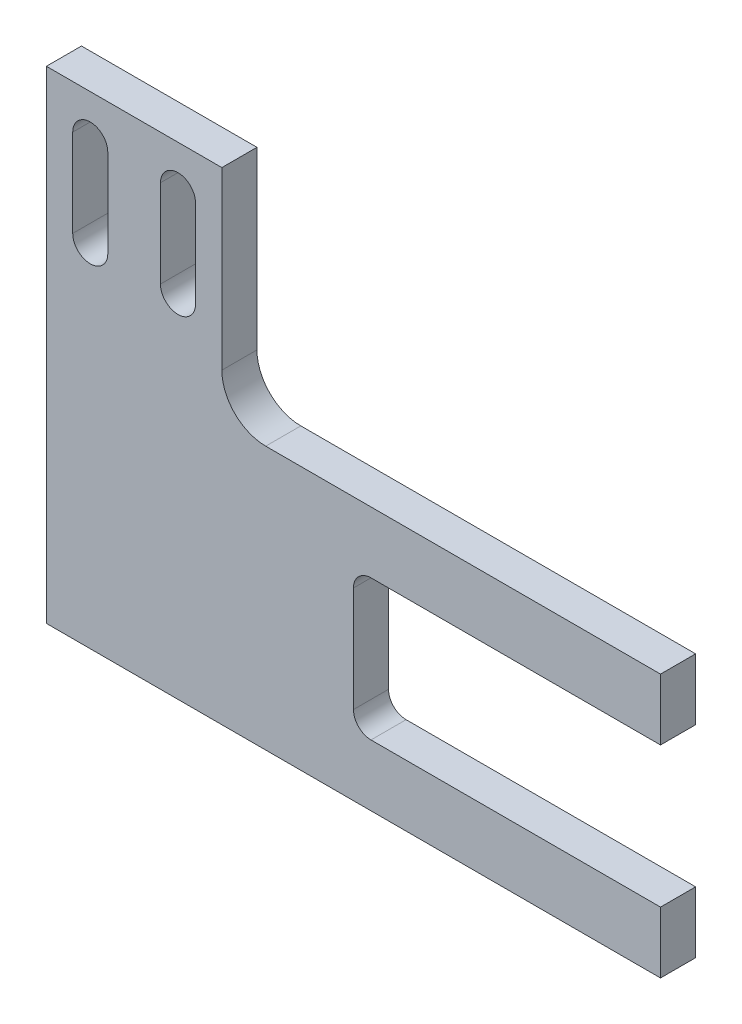
SolidWorks part; units mm, degrees
ref_plane "前视基准面" through (0, 0, 0) normal (0, 0, 1) x (1, 0, 0)
ref_plane "上视基准面" through (0, 0, 0) normal (0, 1, 0) x (1, 0, 0)
ref_plane "右视基准面" through (0, 0, 0) normal (1, 0, 0) x (0, 0, -1)
sketch "草图1" plane through (0, 0, 0) normal (0, 0, 1) x (1, 0, 0)
  line L0 (0, 0) -> (0, -55)
  line L1 (0, -55) -> (70, -55)
  line L2 (70, -55) -> (70, -25)
  line L3 (70, -25) -> (20, -25)
  line L4 (20, -25) -> (20, 0)
  line L5 (20, 0) -> (0, 0)
  dimension "D1" = 20
  dimension "D2" = 30
  dimension "D3" = 25
  dimension "D4" = 50
extrude "凸台-拉伸1" add sketch "草图1" along normal blind 4
sketch "草图2" plane through (0, 0, 4) normal (0, 0, 1) x (1, 0, 0)
  line L0 (5, -15) -> (5, -5) construction
  line L1 (3, -15) -> (3, -5)
  line L2 (7, -15) -> (7, -5)
  line L3 (15, -15) -> (15, -5) construction
  line L4 (13, -15) -> (13, -5)
  line L5 (17, -15) -> (17, -5)
  line L6 (20, -25) -> (20, 0) construction
  line L7 (0, 0) -> (0, -55) construction
  line L8 (20, 0) -> (0, 0) construction
  arc A0 (3, -15) -> (7, -15) centre (5, -15) ccw
  arc A1 (7, -5) -> (3, -5) centre (5, -5) ccw
  arc A2 (13, -15) -> (17, -15) centre (15, -15) ccw
  arc A3 (17, -5) -> (13, -5) centre (15, -5) ccw
  point P2 (5, -10)
  point P8 (15, -10)
  point P14 (0, 0)
  dimension "D1" = 2
  dimension "D2" = 3
  dimension "D3" = 3
  dimension "D4" = 5
  dimension "D5" = 10
extrude "切除-拉伸1" cut sketch "草图2" against normal up to next
fillet "圆角1" radius 5 1 edges at (20, -25, 2)
sketch "草图3" plane through (0, 0, 4) normal (0, 0, 1) x (1, 0, 0)
  line L0 (70, -55) -> (70, -25) construction
  line L1 (70, -32) -> (35, -32)
  line L2 (70, -32) -> (70, -48)
  line L3 (70, -48) -> (35, -48)
  line L4 (35, -32) -> (35, -48)
  line L5 (70, -25) -> (25, -25) construction
  line L6 (0, -55) -> (70, -55) construction
  dimension "D1" = 7
  dimension "D2" = 7
  dimension "D3" = 35
extrude "切除-拉伸2" cut sketch "草图3" against normal up to next
fillet "圆角2" radius 2 2 edges at (35, -48, 2) (35, -32, 2)
